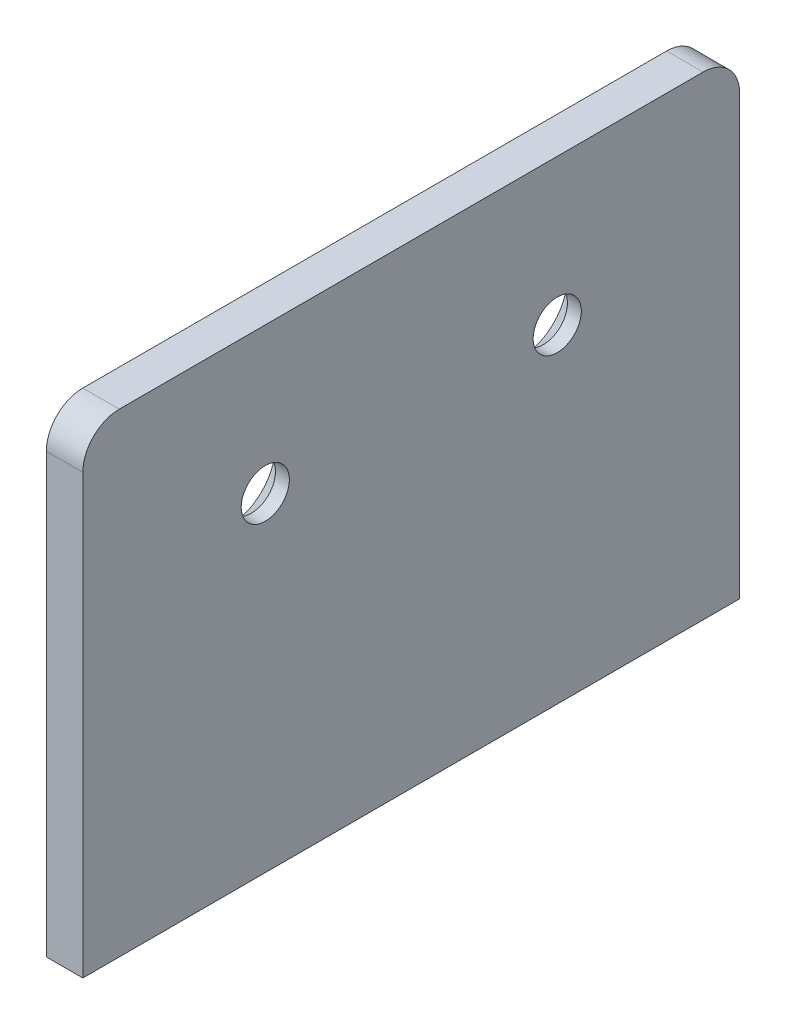
SolidWorks part; units mm, degrees
ref_plane "Front Plane" through (0, 0, 0) normal (0, 0, 1) x (1, 0, 0)
ref_plane "Top Plane" through (0, 0, 0) normal (0, 1, 0) x (1, 0, 0)
ref_plane "Right Plane" through (0, 0, 0) normal (1, 0, 0) x (0, 0, -1)
sketch "Sketch1" plane through (0, 0, 0) normal (1, 0, 0) x (0, 0, -1)
  line L0 (-45, 60) -> (-45, 0)
  line L1 (-45, 0) -> (45, 0)
  line L2 (45, 0) -> (45, 60)
  line L3 (40, 65) -> (-40, 65)
  line L4 (0, 0) -> (0, 65) construction
  arc A0 (-40, 65) -> (-45, 60) centre (-40, 60) ccw
  arc A1 (45, 60) -> (40, 65) centre (40, 60) ccw
  dimension "D3" = 5
  dimension "D4" = 5
  dimension "D1" = 90
  dimension "D2" = 65
extrude "Boss-Extrude1" add sketch "Sketch1" along normal blind 5
hole_wizard "Hole size by hex socket countersunk screw type1" positions "Sketch3" profile "Sketch2" countersink size "M6" standard "GB" end condition through all
sketch "Sketch3" plane through (0, 0, 0) normal (-1, 0, 0) x (0, 0, 1)
  line L0 (-40, 65) -> (40, 65) construction
  point P0 (-20, 45)
  point P1 (20, 45)
  dimension "D1" = 20
  dimension "D2" = 20
  dimension "D3" = 40
  dimension "D4" = 20
sketch "Sketch2" plane through (0, 45, -20) normal (0, 1, 0) x (0, 0, 1)
  line L0 (0, 0) -> (0, 5)
  line L1 (0, 5) -> (3.3, 5)
  line L2 (3.3, 5) -> (3.3, 3.1)
  line L3 (3.3, 3.1) -> (6.4, 0)
  line L5 (6.4, 0) -> (0, 0)
  line L6 (-3.3, 3.1) -> (-6.4, 0) construction
  line L11 (0, -6.35) -> (0, 107.95) construction
  dimension "通孔孔直径" = 6.6
  dimension "通孔孔深度" = 5
  dimension "近端锥形沉头孔直径" = 12.8
  dimension "近端锥形沉头孔角度" = 90
